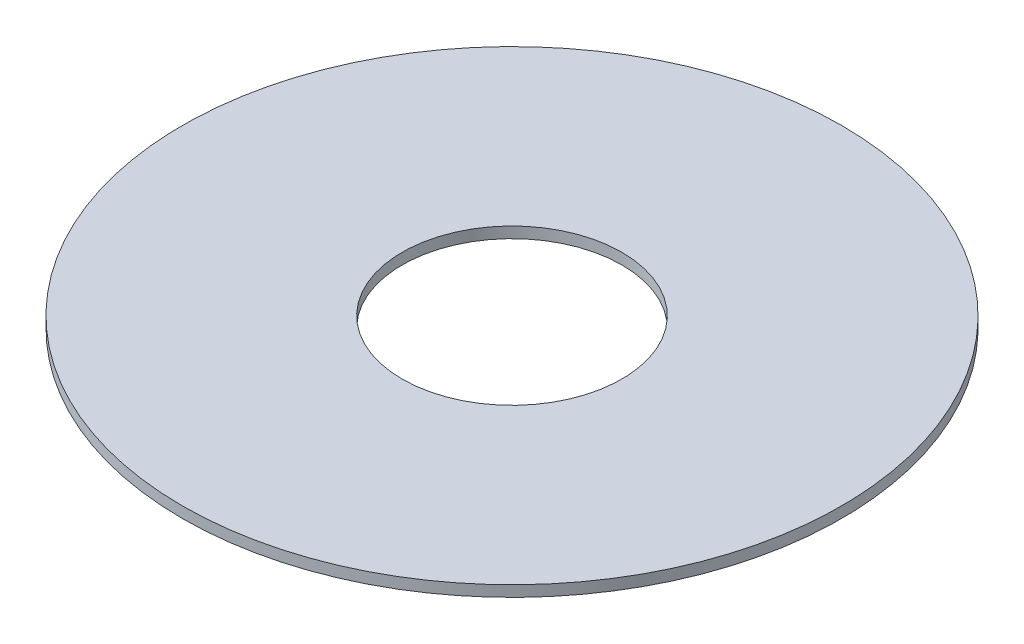
SolidWorks part; units mm, degrees
ref_plane "Front Plane" through (0, 0, 0) normal (0, 0, 1) x (1, 0, 0)
ref_plane "Top Plane" through (0, 0, 0) normal (0, 1, 0) x (1, 0, 0)
ref_plane "Right Plane" through (0, 0, 0) normal (1, 0, 0) x (0, 0, -1)
other "Configuration Table"
sketch "Sketch1" plane through (0, 0, 0) normal (0, 1, 0) x (1, 0, 0)
  circle A0 centre (0, 0) radius 20
  circle A1 centre (0, 0) radius 60
  dimension "D1" = 120
  dimension "D2" = 40
extrude "Boss-Extrude1" add sketch "Sketch1" along normal blind 2
